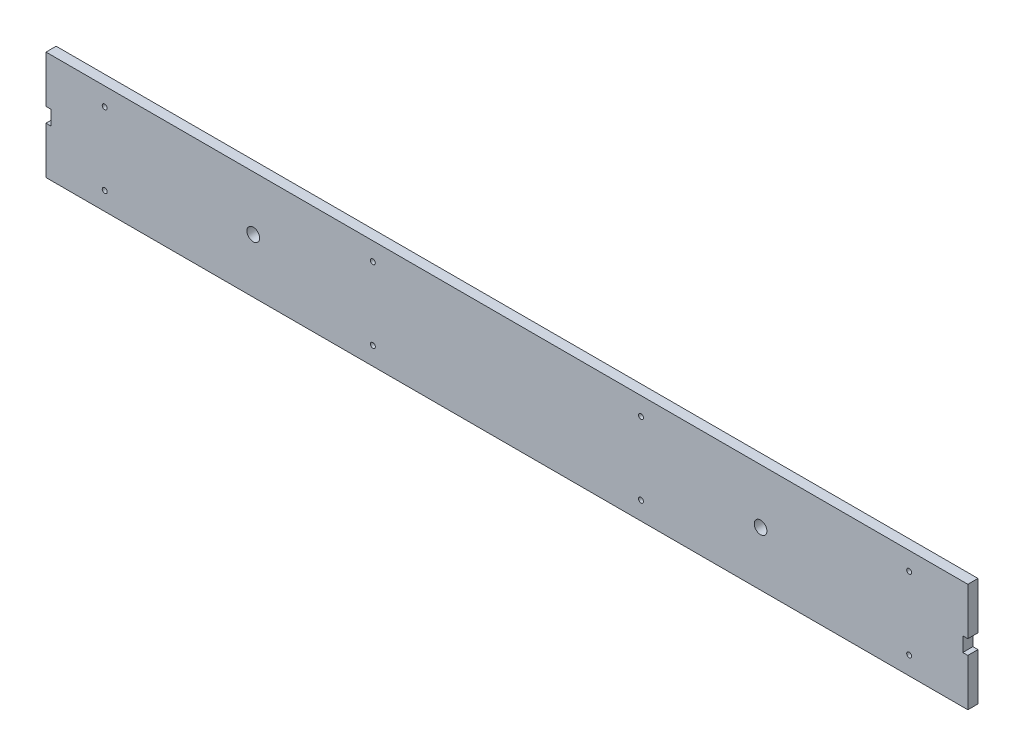
SolidWorks part; units mm, degrees
material "Q235"
ref_plane "Front Plane" through (0, 0, 0) normal (0, 0, 1) x (1, 0, 0)
ref_plane "Top Plane" through (0, 0, 0) normal (0, 1, 0) x (1, 0, 0)
ref_plane "Right Plane" through (0, 0, 0) normal (1, 0, 0) x (0, 0, -1)
sketch "Sketch1" plane through (0, 0, 0) normal (0, 0, 1) x (1, 0, 0)
  line L0 (0, 75) -> (1272, 75) construction
  line L1 (0, 0) -> (1272, 0)
  line L2 (0, 0) -> (0, 150)
  line L3 (0, 150) -> (1272, 150)
  line L4 (1272, 0) -> (1272, 150)
  line L5 (636, 150) -> (636, 0) construction
  circle A0 centre (286, 75) radius 8.75
  circle A1 centre (986, 75) radius 8.75
  dimension "D4" = 17.5
  dimension "D1" = 150
  dimension "D2" = 1272
  dimension "D5" = 350
  dimension "D6" = 350
extrude "Boss-Extrude1" add sketch "Sketch1" along normal blind 14
hole_wizard "M8 Tapped Hole1" positions "3DSketch1" profile "Sketch2" tap size "M8" standard "GB" end condition through all
sketch3d "3DSketch1"
  line L0 (81, 125, 14) -> (81, 25, 14) construction
  line L1 (81, 25, 14) -> (1191, 25, 14) construction
  line L2 (1191, 25, 14) -> (1191, 125, 14) construction
  line L3 (1191, 125, 14) -> (81, 125, 14) construction
  line L5 (451, 125, 14) -> (451, 25, 14) construction
  line L7 (821, 125, 14) -> (821, 25, 14) construction
  line L11 (1272, 150, 14) -> (0, 150, 14) construction
  line L12 (0, 0, 14) -> (1272, 0, 14) construction
  line L13 (636, 150, 14) -> (636, 0, 14) construction
  point P0 (81, 125, 14)
  point P2 (81, 25, 14)
  point P4 (451, 125, 14)
  point P6 (451, 25, 14)
  point P8 (821, 125, 14)
  point P10 (821, 25, 14)
  point P12 (1191, 125, 14)
  point P14 (1191, 25, 14)
  dimension "D1" = 370
  dimension "D2" = 185
  dimension "D3" = 25
  dimension "D4" = 25
  dimension "D5" = 370
  dimension "D6" = 370
sketch "Sketch2" plane through (81, 125, 14) normal (1, 0, 0) x (0, -1, 0)
  line L0 (0, 0) -> (0, 14)
  line L1 (0, 14) -> (3.4, 14)
  line L2 (3.4, 14) -> (3.4, 0)
  line L5 (3.4, 0) -> (0, 0)
  line L11 (0, -6.35) -> (0, 107.95) construction
  dimension "通孔螺纹孔钻头直径" = 6.8
  dimension "通孔螺纹孔钻头深度" = 14
cosmetic thread "Cosmetic Thread1" parameters "D2"=8
cosmetic thread "Cosmetic Thread2" parameters "D2"=8
cosmetic thread "Cosmetic Thread3" parameters "D2"=8
cosmetic thread "Cosmetic Thread4" parameters "D2"=8
cosmetic thread "Cosmetic Thread5" parameters "D2"=8
cosmetic thread "孔螺蚊线6" parameters "D2"=8
cosmetic thread "孔螺蚊线7" parameters "D2"=8
cosmetic thread "孔螺蚊线8" parameters "D2"=8
sketch "Sketch5" plane through (0, 0, 14) normal (0, 0, 1) x (1, 0, 0)
  line L0 (0, 150) -> (0, 0) construction
  line L1 (-7, 85) -> (7, 85)
  line L2 (-7, 85) -> (-7, 65)
  line L3 (-7, 65) -> (7, 65)
  line L4 (7, 85) -> (7, 65)
  line L5 (-7, 85) -> (7, 65) construction
  line L6 (-7, 65) -> (7, 85) construction
  line L7 (1272, 0) -> (1272, 150) construction
  line L8 (1265, 85) -> (1279, 85)
  line L9 (1265, 85) -> (1265, 65)
  line L10 (1265, 65) -> (1279, 65)
  line L11 (1279, 85) -> (1279, 65)
  line L12 (1265, 85) -> (1279, 65) construction
  line L13 (1265, 65) -> (1279, 85) construction
  point P0 (0, 75)
  point P7 (1272, 75)
  dimension "D1" = 14
  dimension "D2" = 20
  dimension "D3" = 14
  dimension "D4" = 20
extrude "Cut-Extrude1" cut sketch "Sketch5" against normal through all
